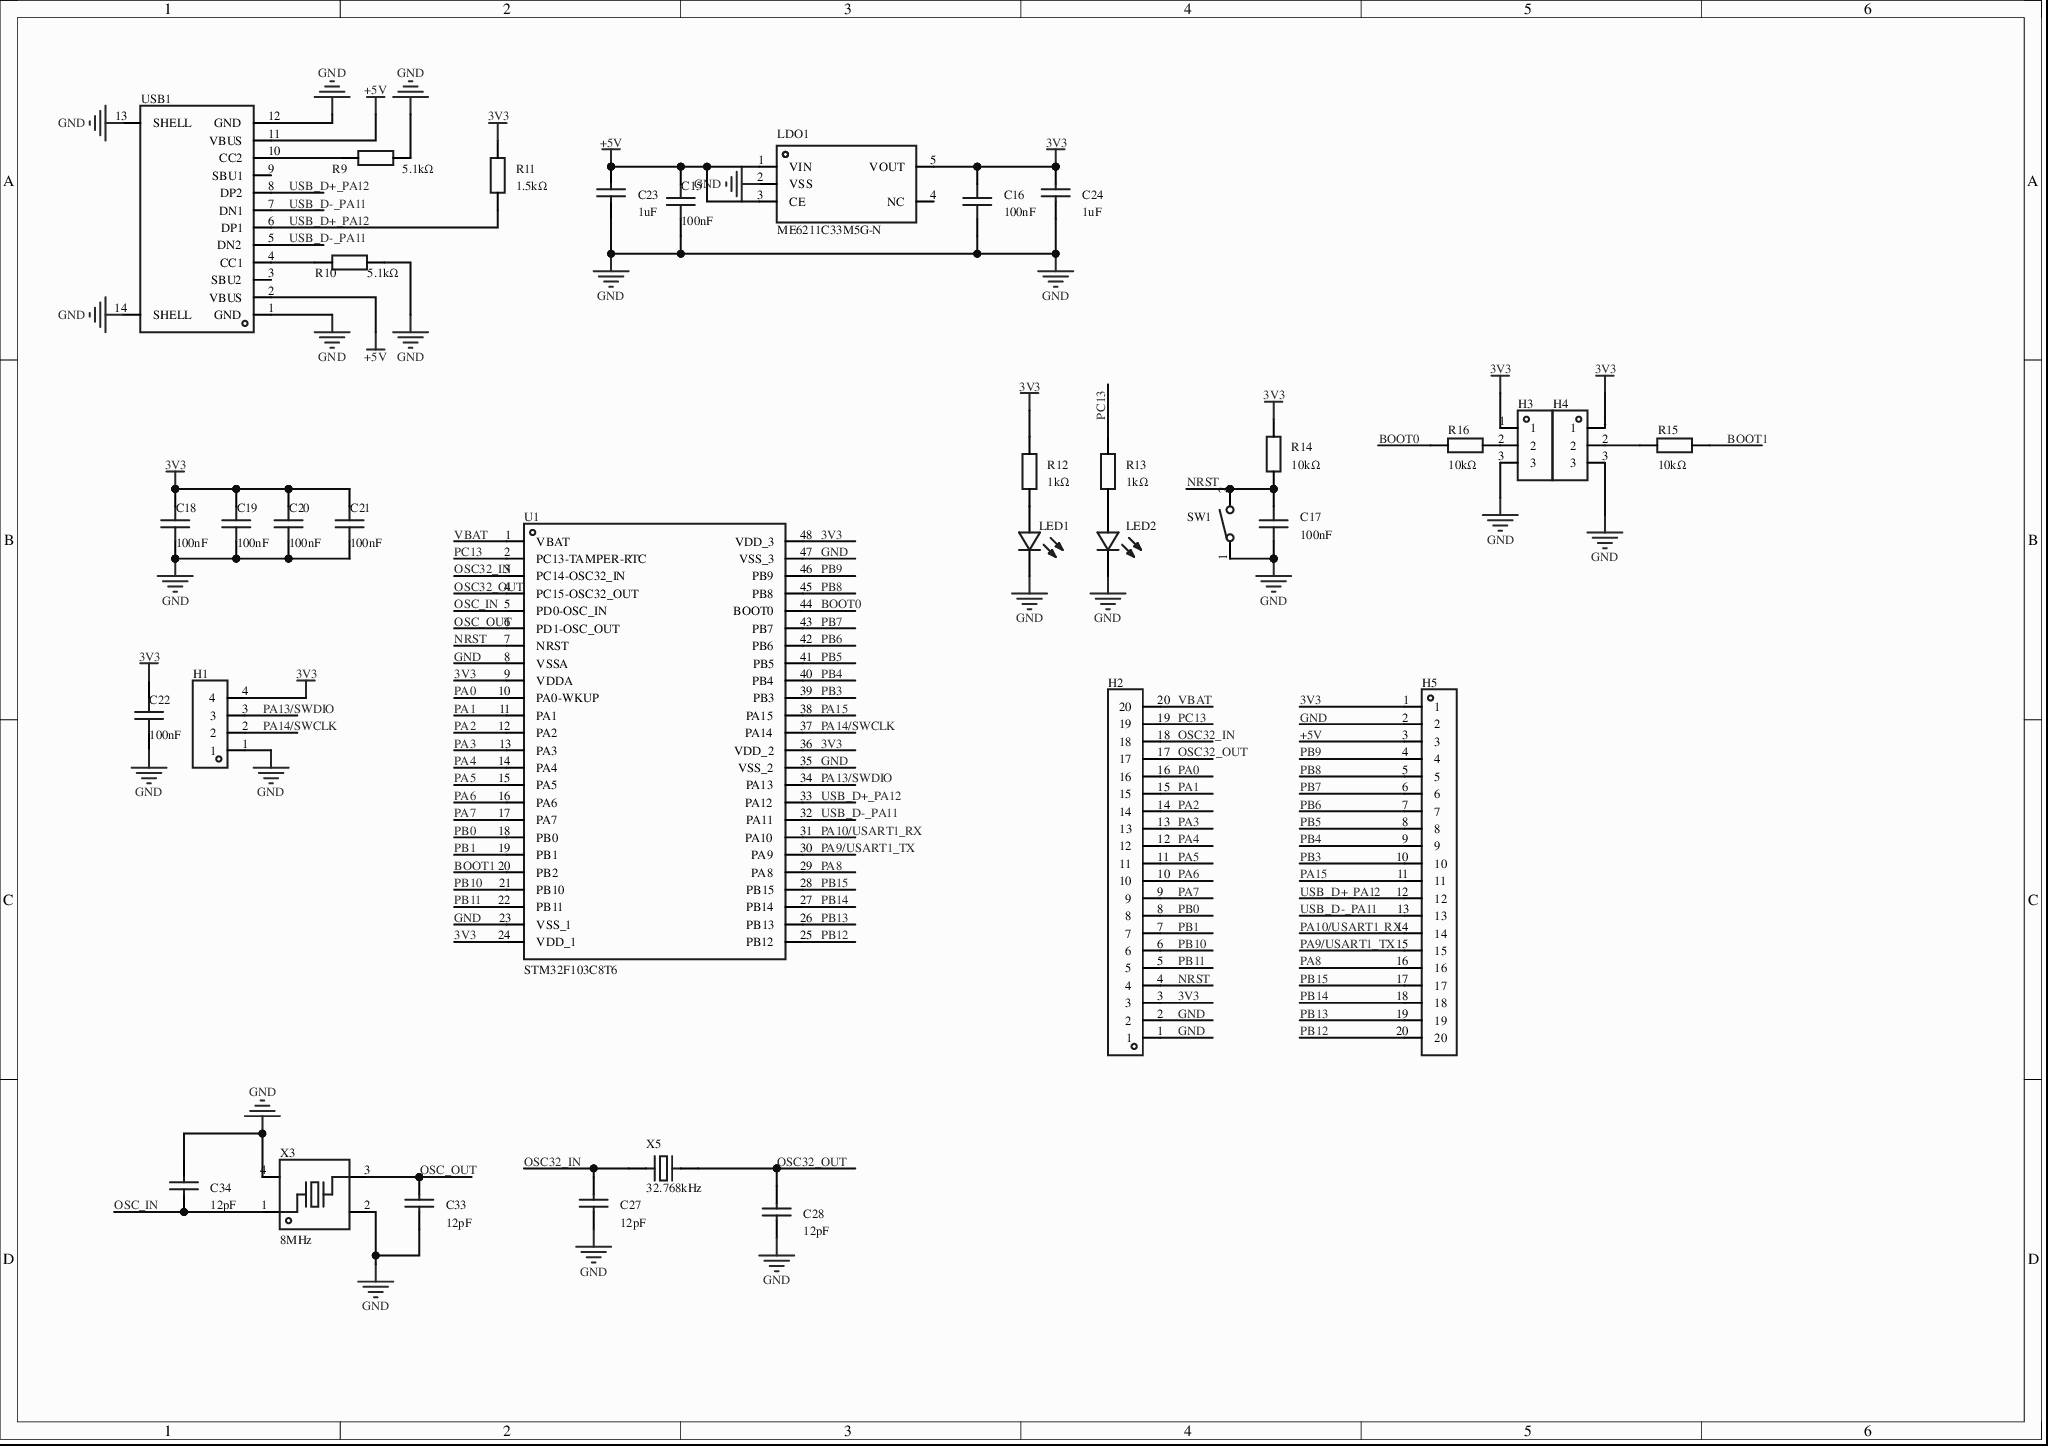
[diagram p0: MISC51884-3.schdoc]
# Altium project MISC51884-2.PrjPcb
1 sheet, 35 parts. Net scope: global (net labels, ports and power ports of the same name join across sheets).
Board file: MISC51884.pcbdoc

## Sheet MISC51884-3.schdoc
size 297 x 209 mm; Version: V1.0; @Project Name: MISC51884; @Update Date: 2026-04-17; @Create Date: 2026-04-17; @Board Name: MISC51884; @Create Time: 21:12:34; @Page Count: 1; @Page No: 1; @Schematic Name: MISC51884; @Update Time: 21:12:34; Size: A4

### Parts
C15  100nF  [C0402]
C16  100nF  [C0402]
C17  100nF  [C0402]
C18  100nF  [C0402]
C19  100nF  [C0402]
C20  100nF  [C0402]
C21  100nF  [C0402]
C22  100nF  [C0402]
C23  1uF  [C0402]
C24  1uF  [C0402]
C27  12pF  [C0402]
C28  12pF  [C0402]
C33  12pF  [C0402]
C34  12pF  [C0402]
H1  DZ254W-11-04-65  [HDR-TH_4P-P2.54-H-M-W10.3]  (value not drawn)
H2  2.54-1*20P直针  [HDR-TH_20P-P2.54-V-M-1]  (value not drawn)
H3  PZ254V-11-03P  [HDR-TH_3P-P2.54-V-M_PZ254V-11-03P]  (value not drawn)
H4  PZ254V-11-03P  [HDR-TH_3P-P2.54-V-M_PZ254V-11-03P]  (value not drawn)
H5  2.54-1*20P直针  [HDR-TH_20P-P2.54-V-M-1]  (value not drawn)
LDO1  ME6211C33M5G-N  [SOT-23-5_L3.0-W1.7-P0.95-LS2.8-BL]
LED1  NCD0603R1  [LED0603-RD_RED]  (value not drawn)
LED2  NCD0603B1  [LED0603-RD]  (value not drawn)
R9  5.1kΩ  [R0805]
R10  5.1kΩ  [R0805]
R11  1.5kΩ  [R0805]
R12  1kΩ  [R0805]
R13  1kΩ  [R0805]
R14  10kΩ  [R0805]
R15  10kΩ  [R0805]
R16  10kΩ  [R0805]
SW1  TS-1101-B-W  [KEY-SMD_2P-L6.0-W3.6-P7.4-LS8.0-L]  (value not drawn)
U1  STM32F103C8T6  [LQFP-48_L7.0-W7.0-P0.50-LS9.0-BL]
USB1  TYPE-C 16PIN 2MD(073)  [USB-C-SMD_TYPE-C-6PIN-2MD-073]  (value not drawn)
X3  8MHz  [CRYSTAL-SMD_4P-L3.2-W2.5-BL-1]
X5  32.768kHz  [OSC-SMD_L3.2-W1.5]

### Nets
3V3: C16.2 C18.2 C19.2 C20.2 C21.2 C22.2 C24.2 H1.4 H2.3 H3.1 H4.1 H5.1 LDO1.5(VOUT) R11.2 R12.2 R14.2 U1.9(VDDA) U1.24(VDD_1) U1.36(VDD_2) U1.48(VDD_3)
+5V: C15.2 C23.2 H5.3 LDO1.1(VIN) LDO1.3(CE) USB1.2(VBUS) USB1.11(VBUS)
GND: C15.1 C16.1 C17.1 C18.1 C19.1 C20.1 C21.1 C22.1 C23.1 C24.1 C27.1 C28.1 C33.1 C34.2 H1.1 H2.1 H2.2 H3.3 H4.3 H5.2 LDO1.2(VSS) LED1.1(K) LED2.1(-) R9.2 R10.2 SW1.1 U1.8(VSSA) U1.23(VSS_1) U1.35(VSS_2) U1.47(VSS_3) USB1.1(GND) USB1.12(GND) USB1.13(SHELL) USB1.14(SHELL) X3.2(GND) X3.4(GND)
BOOT0: R16.1 U1.44(BOOT0)
BOOT1: R15.2 U1.20(PB2)
NRST: C17.2 H2.4 R14.1 SW1.2 U1.7(NRST)
OSC32_IN: C27.2 H2.18 U1.3(PC14-OSC32_IN) X5.1
OSC32_OUT: C28.2 H2.17 U1.4(PC15-OSC32_OUT) X5.2
OSC_IN: C34.1 U1.5(PD0-OSC_IN) X3.1
OSC_OUT: C33.2 U1.6(PD1-OSC_OUT) X3.3
PA0: H2.16 U1.10(PA0-WKUP)
PA1: H2.15 U1.11(PA1)
PA2: H2.14 U1.12(PA2)
PA3: H2.13 U1.13(PA3)
PA4: H2.12 U1.14(PA4)
PA5: H2.11 U1.15(PA5)
PA6: H2.10 U1.16(PA6)
PA7: H2.9 U1.17(PA7)
PA8: H5.16 U1.29(PA8)
PA9/USART1_TX: H5.15 U1.30(PA9)
PA10/USART1_RX: H5.14 U1.31(PA10)
PA13/SWDIO: H1.3 U1.34(PA13)
PA14/SWCLK: H1.2 U1.37(PA14)
PA15: H5.11 U1.38(PA15)
PB0: H2.8 U1.18(PB0)
PB1: H2.7 U1.19(PB1)
PB3: H5.10 U1.39(PB3)
PB4: H5.9 U1.40(PB4)
PB5: H5.8 U1.41(PB5)
PB6: H5.7 U1.42(PB6)
PB7: H5.6 U1.43(PB7)
PB8: H5.5 U1.45(PB8)
PB9: H5.4 U1.46(PB9)
PB10: H2.6 U1.21(PB10)
PB11: H2.5 U1.22(PB11)
PB12: H5.20 U1.25(PB12)
PB13: H5.19 U1.26(PB13)
PB14: H5.18 U1.27(PB14)
PB15: H5.17 U1.28(PB15)
PC13: H2.19 R13.2 U1.2(PC13-TAMPER-RTC)
USB_D+_PA12: H5.12 R11.1 U1.33(PA12) USB1.6(DP1) USB1.8(DP2)
USB_D-_PA11: H5.13 U1.32(PA11) USB1.5(DN2) USB1.7(DN1)
VBAT: H2.20 U1.1(VBAT)
NetH3_2: H3.2 R16.2
NetH4_2: H4.2 R15.1
NetLED1_2: LED1.2(A) R12.1
NetLED2_2: LED2.2(+) R13.1
NetR9_1: R9.1 USB1.10(CC2)
NetR10_1: R10.1 USB1.4(CC1)

Not connected (* = marked no-connect by the designer): LDO1 4(NC)*; USB1 3(SBU2)* 9(SBU1)*

### Library data of the parts
C15-C22 = GRM155R71H104KE14D: 容值:100nF;精度:±10%;额定电压:50V;温度系数:X7R;; Manufacturer: muRata(村田); AddInBom: yes; ModelId: 36a51122f27c49738f86b3bfa98863e00819f05c4eef4c71ace90d822a990e87; ModelName: C0402_L1.0-W0.5-H0.5; ModelTransform: 39.37,19.685,0,0,0,0,0,0,0; Tolerance: ±10%; Voltage Rating: 50V; Temperature Coefficient: X7R; Symbol: GRM155R71H104KE14D; Device: GRM155R71H104KE14D; LCSC Part Name: 100nF ±10% 50V; SupplierPart: C77020; ManufacturerPart: GRM155R71H104KE14D; Supplier Footprint: 0402; JLCPCB Part Class: Extended Part; Datasheet: https://item.szlcsc.com/datasheet/GRM155R71H104KE14D/78147.html; Supplier: LCSC; ConvertToPcb: yes; FootprintName: C0402; Value: 100nF
C23 C24 = CL05A105KP5NNNC: 容值:1uF;精度:±10%;额定电压:10V;温度系数:X5R;; Manufacturer: SAMSUNG(三星); AddInBom: yes; ModelId: 36a51122f27c49738f86b3bfa98863e00819f05c4eef4c71ace90d822a990e87; ModelName: C0402_L1.0-W0.5-H0.5; ModelTransform: 39.37,19.685,0,0,0,0,0,0,0; Tolerance: ±10%; Voltage Rating: 10V; Temperature Coefficient: X5R; Symbol: CL05A105KP5NNNC; Device: CL05A105KP5NNNC; LCSC Part Name: 1uF ±10% 10V; SupplierPart: C14445; ManufacturerPart: CL05A105KP5NNNC; Supplier Footprint: 0402; JLCPCB Part Class: Extended Part; Datasheet: https://item.szlcsc.com/datasheet/CL05A105KP5NNNC/15107.html; Supplier: LCSC; ConvertToPcb: yes; FootprintName: C0402; Value: 1uF
C27 C28 C33 C34 = 0402CG120J500NT: 容值:12pF;精度:±5%;额定电压:50V;温度系数:C0G;; Manufacturer: FH(风华); AddInBom: yes; ModelId: 36a51122f27c49738f86b3bfa98863e00819f05c4eef4c71ace90d822a990e87; ModelName: C0402_L1.0-W0.5-H0.5; ModelTransform: 39.37,19.685,0,0,0,0,0,0,0; Tolerance: ±5%; Voltage Rating: 50V; Temperature Coefficient: C0G; Symbol: 0402CG120J500NT; Device: 0402CG120J500NT; LCSC Part Name: 12pF ±5% 50V; SupplierPart: C1547; ManufacturerPart: 0402CG120J500NT; Supplier Footprint: 0402; JLCPCB Part Class: Basic Part; Datasheet: https://item.szlcsc.com/datasheet/0402CG120J500NT/1899.html; Supplier: LCSC; ConvertToPcb: yes; FootprintName: C0402; Value: 12pF
H1 = DZ254W-11-04-65: 插针结构:1x4P;间距:2.54mm;行距:-;圆针/方针:方针;安装方式:弯插;排数:单排;总PIN位数:4P;额定电流:3A;额定电压:-;配合针长度:6mm;塑高:2.54mm;端接针长度:-;触头材质:黄铜;触头镀层:金;工作温度:-;颜色:黑色;; Manufacturer: DEALON(德艺隆); AddInBom: yes; ModelId: 380738e2c3344fc1a10fb2457d15d4660819f05c4eef4c71ace90d822a990e87; ModelTransform: 400.003,407.873,0,180,0,0,0,191.299,-118.11; Pin Structure: 1x4P; Pitch: 2.54mm; Circluar Pins/Square Pins: 方针; Current Rating: 3A; Symbol: DZ254W-11-04-65; Device: DZ254W-11-04-65; LCSC Part Name: 1x4P 间距:2.54mm 方针 弯插; SupplierPart: C2935929; ManufacturerPart: DZ254W-11-04-65; Supplier Footprint: 弯插,P=2.54mm; JLCPCB Part Class: Extended Part; Datasheet: https://item.szlcsc.com/datasheet/DZ254W-11-04-65/3287507.html; Supplier: LCSC; ConvertToPcb: yes; FootprintName: HDR-TH_4P-P2.54-H-M-W10.3; ModelName: HDR-TH_4P-P2.54-H-M-W10.3; Row Spacing: -; Mounting Type: 弯插; Number of Rows: 单排; Number of Pins: 4P; Voltage Rating (Max): -; Length of Mating Pin: 6mm; Insulation Height: 2.54mm; Length of End Connection Pin: -; Contact Material: 黄铜; Contact Plating: 金; Operating Temperature: -; Color: 黑色
H2 H5 = 2.54-1*20P直针: 插针结构:1x20P;间距:2.54mm;行距:-;圆针/方针:方针;安装方式:直插;排数:单排;总PIN位数:20P;额定电流:3A;额定电压:-;配合针长度:-;塑高:-;端接针长度:-;触头材质:黄铜;触头镀层:-;工作温度:-40℃~+105℃;颜色:黑色;; Manufacturer: BOOMELE(博穆精密); Symbol: Header-Male-2.54_1x20; AddInBom: yes; ModelId: f68709be121d406db68b06f32a5953890819f05c4eef4c71ace90d822a990e87; ModelName: HDR-M-2.54_1x20; ModelTransform: 1999.996,100,0,0,0,0,0,0,-118.11; Pin Structure: 1x20P; Pitch: 2.54mm; Circluar Pins/Square Pins: 方针; Current Rating: 3A; Device: 2.54-1*20P直针; LCSC Part Name: 1x20P 间距:2.54mm 方针 直插; SupplierPart: C50981; ManufacturerPart: 2.54-1*20P直针; Supplier Footprint: 插件,P=2.54mm; JLCPCB Part Class: Extended Part; Datasheet: https://item.szlcsc.com/datasheet/2.54-1*20P%25E7%259B%25B4%25E9%2592%2588/51993.html; Supplier: LCSC; ConvertToPcb: yes; FootprintName: HDR-TH_20P-P2.54-V-M-1; Row Spacing: -; Mounting Type: 直插; Number of Rows: 单排; Number of Pins: 20P; Voltage Rating (Max): -; Length of Mating Pin: -; Insulation Height: -; Length of End Connection Pin: -; Contact Material: 黄铜; Contact Plating: -; Operating Temperature: -40℃~+105℃; Color: 黑色
H3 H4 = PZ254V-11-03P: 插针结构:1x3P;间距:2.54mm;行距:-;圆针/方针:方针;安装方式:直插;排数:单排;总PIN位数:3P;额定电流:3A;额定电压:250V;配合针长度:6mm;塑高:2.5mm;端接针长度:3mm;工作温度:-40℃~+105℃;颜色:黑色;; Manufacturer: XFCN(兴飞); Symbol: PZ254V-11-03P_C2937625; 3D Model: bd28a638fbd247be9398fd5d39c366ec0819f05c4eef4c71ace90d822a990e87; 3D Model Transform: 300.3931,100,0,0,0,0,0,0,-118.11; Pin Structure: 1x3P; Pitch: 2.54mm; Circluar Pins/Square Pins: 方针; Current Rating: 3A; Voltage Rating (Max): 250V; AddInBom: yes; Device: PZ254V-11-03P; LCSC Part Name: 1x3P 间距:2.54mm 方针 直插; Supplier Part: C2937625; Manufacturer Part: PZ254V-11-03P; Supplier Footprint: 插件,P=2.54mm; JLCPCB Part Class: Extended Part; Datasheet: https://item.szlcsc.com/datasheet/PZ254V-11-03P/3293280.html; Supplier: LCSC; Row Spacing: -; Mounting Type: 直插; Number of Rows: 单排; Number of Pins: 3P; Length of Mating Pin: 6mm; Insulation Height: 2.5mm; Length of End Connection Pin: 3mm; Operating Temperature: -40℃~+105℃; Color: 黑色; ConvertToPcb: yes; FootprintName: HDR-TH_3P-P2.54-V-M_PZ254V-11-03P; ModelName: HDR-TH_3P-P2.54-V-M_PZ254V-11-03P
LDO1 = ME6211C33M5G-N: 输出类型:固定;工作电压:6V;输出电压:3.3V;输出电流:500mA;电源纹波抑制比(PSRR):70dB@(1kHz);输出极性:正极;; Manufacturer: MICRONE(南京微盟); 3D Model: 0a2a1b8f50944f73965918ad6e5fe1670819f05c4eef4c71ace90d822a990e87; 3D Model Transform: 118.60433,114.173,0,90,0,0,0.0005,0.0005,0; Output Type: 固定; Voltage - Supply: 6V; Output Voltage: 3.3V; Output Current: 500mA; Voltage Dropout: 120mV@(100mA); standby current: 60uA; Noise: 50uVrms; Output Configuration: 正极; Number of Outputs: 1; AddInBom: yes; ModelName: SOT-23-5_L2.9-W1.6-H1.1-LS2.8-P0.95; Symbol: ME6211C33M5G-N; Device: ME6211C33M5G-N; LCSC Part Name: 输入6V 输出3.3V 500mA; Supplier Part: C82942; Manufacturer Part: ME6211C33M5G-N; Supplier Footprint: SOT-23-5; JLCPCB Part Class: Extended Part; Datasheet: https://item.szlcsc.com/datasheet/ME6211C33M5G-N/84106.html; Supplier: LCSC; Power Supply Rejection Ratio (PSRR): 70dB@(1kHz); Features: 过流保护；带使能；短路保护; Operating Temperature: -40℃~+150℃; ConvertToPcb: yes; FootprintName: SOT-23-5_L3.0-W1.7-P0.95-LS2.8-BL
LED1 = NCD0603R1_C84263: 灯头类型:-;发光颜色:红色;正向压降(Vf):1.6V~2.6V;功率:65mW;正向电流:25mA;波长:615nm~630nm;二极管配置:独立二极管;透镜颜色:-;色温:-;发光强度:220mcd;发光角度:130°;载带方式:-;工作温度:-30℃~+85℃;; Manufacturer: 国星光电; Symbol: FC-DA1608HRK-620D; AddInBom: yes; ModelId: 74041d3a270d435c8600a9ab9b7641c00819f05c4eef4c71ace90d822a990e87; ModelTransform: 63.7794,31.496,0,0,0,0,0,-0.002,0; Illumination Color: 红色; Power(Watts): 65mW; Forward Current: 25mA; Peak Wavelength: 630nm; Diode Configuration: 独立二极管; Luminous Intensity: 220mcd; Viewing Angle: 130°; Device: NCD0603R1_C84263; LCSC Part Name: 片式发光二极管; SupplierPart: C84263; ManufacturerPart: NCD0603R1; Supplier Footprint: 0603; JLCPCB Part Class: Extended Part; Datasheet: https://item.szlcsc.com/datasheet/NCD0603R1/85432.html; Supplier: LCSC; ConvertToPcb: yes; FootprintName: LED0603-RD_RED; ModelName: LED0603-RD_RED; Lamp Holder Type: -; Voltage - Forward(Vf): 1.6V~2.6V; Wavelength - Dominant: 615nm~630nm; Lens Color: -; Color Temperature: -; Mounting Style: -; Operating Temperature: -30℃~+85℃
LED2 = NCD0603B1: 灯头类型:-;发光颜色:蓝色;正向压降(Vf):2.6V~3.6V;功率:72mW;正向电流:10mA;波长:463nm~475nm;二极管配置:独立二极管;透镜颜色:-;色温:-;发光强度:220mcd;发光角度:130°;载带方式:-;工作温度:-30℃~+85℃;; Manufacturer: 国星光电; Symbol: FC-DA1608BK-470H10; AddInBom: yes; ModelId: 1f0d29a91be547639d425604e9b96ebb0819f05c4eef4c71ace90d822a990e87; ModelTransform: 63.7794,32.283,0,0,0,0,0,0,0; Illumination Color: 蓝色; Power(Watts): 72mW; Forward Current: 10mA; Peak Wavelength: 465nm; Diode Configuration: 独立二极管; Luminous Intensity: 220mcd; Viewing Angle: 130°; Device: NCD0603B1; LCSC Part Name: 片式发光二极管; SupplierPart: C84266; ManufacturerPart: NCD0603B1; Supplier Footprint: 0603; JLCPCB Part Class: Extended Part; Datasheet: https://item.szlcsc.com/datasheet/NCD0603B1/85435.html; Supplier: LCSC; ConvertToPcb: yes; FootprintName: LED0603-RD; ModelName: LED0603-RD; Lamp Holder Type: -; Voltage - Forward(Vf): 2.6V~3.6V; Wavelength - Dominant: 463nm~475nm; Lens Color: -; Color Temperature: -; Mounting Style: -; Operating Temperature: -30℃~+85℃
R9-R16 = Res_0805: Symbol: 电阻; ConvertToPcb: yes; ModelId: 37a81e68749a4138bd2dfa6897b24b850819f05c4eef4c71ace90d822a990e87; ModelName: R0805_L2.0-W1.3-H0.6; ModelTransform: 78.74,51.181,0,0,0,0,0,-0.0005,0; Device: Res_0805; AddInBom: yes; Supplier Footprint: 0805; FootprintName: R0805
  R9 R10: Value: 5.1kΩ
  R11: Value: 1.5kΩ
  R12 R13: Value: 1kΩ
  R14-R16: Value: 10kΩ
SW1 = TS-1101-B-W_C500065: 电路结构:单刀单掷;按钮形状:矩形按钮;作用力:1.6N;安装方式:立贴;开关长度:6mm;开关宽度:3.6mm;开关高度:2.5mm;带支架:不带支架;触点电流:50mA;额定电压:12V;带灯:无;工作寿命:5万次;; Manufacturer: XKB Connection(中国星坤); AddInBom: yes; ModelId: b8d6ee452e6447ebb6dcd7a0adaffe040819f05c4eef4c71ace90d822a990e87; ModelTransform: 314.96,141.732,0,0,0,0,0,0,0; Circuit: 单刀单掷; Actuator Style: 矩形按钮; Operating Force: 1.6N; Switch Height: 2.5mm; with Bracket: 不带支架; Contact Current: 50mA; Voltage Rating: 12V; Actuator/Cap Color: 白色; With Lamp: 无; Life: 5万次; Symbol: TS-1101-B-W; Device: TS-1101-B-W_C500065; LCSC Part Name: 6*3.6*2.5mm 立贴 轻触开关; SupplierPart: C500065; ManufacturerPart: TS-1101-B-W; Supplier Footprint: SMD; JLCPCB Part Class: Extended Part; Datasheet: https://item.szlcsc.com/datasheet/TS-1101-B-W/512191.html; Supplier: LCSC; ConvertToPcb: yes; FootprintName: KEY-SMD_2P-L6.0-W3.6-P7.4-LS8.0-L; ModelName: KEY-SMD_2P-L6.0-W3.6-P7.4-LS8.0-L; Mounting Type: 立贴; Length: 6mm; Width: 3.6mm; Operating Temperature: -30℃~+85℃
U1 = STM32F103C8T6: CPU内核:ARM-M3;CPU最大主频:72MHz;应用领域:-;; Manufacturer: ST(意法半导体); AddInBom: yes; ModelId: 093be70396ff421eb2cdb946d5311efc0819f05c4eef4c71ace90d822a990e87; ModelName: LQFP-48_L7.0-W7.0-H1.4-LS9.0-P0.50; ModelTransform: 354.331,354.331,0,0,0,0,0,0,0; CPU Core: ARM-M3; CPU Maximum Speed: 72MHz; Program Storage Size: 64KB; Program Memory Type: FLASH; Number of I/O: 37; ADC (Bit): 12bit; Voltage - Supply: 2V~3.6V; Symbol: STM32F103C8T6; Device: STM32F103C8T6; LCSC Part Name: 主流增强型ARM Cortex-M3 MCU，具有64 KB Flash、72 MHz CPU、电机控制、USB和CAN; SupplierPart: C8734; ManufacturerPart: STM32F103C8T6; Supplier Footprint: LQFP-48(7x7); JLCPCB Part Class: Extended Part; Datasheet: https://item.szlcsc.com/datasheet/STM32F103C8T6/9243.html; Supplier: LCSC; ConvertToPcb: yes; FootprintName: LQFP-48_L7.0-W7.0-P0.50-LS9.0-BL; Applications: -
USB1 = TYPE-C 16PIN 2MD(073): 连接器类型:Type-C;协议标准:-;公母:母;安装方式:卧贴;触点数量:16P;端口数量:1;额定电流 - 电源:3A;工作温度:-25℃~+85℃;; Manufacturer: SHOU HAN(首韩); AddInBom: yes; ModelId: 3a41b9ec9b654a0fad4d118405ec62900819f05c4eef4c71ace90d822a990e87; ModelTransform: 351.9678,298.4246,0,0,0,0,0,-47.244,-35.433; Gender: 母; Number of Contacts: 16P; Number of Ports: 1; Current Rating-Power: 3A; Voltage Rating: 5V; Connect-Disconnect Life: 1万次; Detection color: 黑色; Symbol: TYPE-C 16PIN 2MD(073); Device: TYPE-C 16PIN 2MD(073); LCSC Part Name: Type-C 母 卧贴; SupplierPart: C2765186; ManufacturerPart: TYPE-C 16PIN 2MD(073); Supplier Footprint: SMD; JLCPCB Part Class: Extended Part; Datasheet: https://item.szlcsc.com/datasheet/TYPE-C%252016PIN%25202MD(073)/2901843.html; Supplier: LCSC; ConvertToPcb: yes; FootprintName: USB-C-SMD_TYPE-C-6PIN-2MD-073; ModelName: USB-C-SMD_TYPE-C-6PIN-2MD-073; Connector Type: Type-C; Protocol Standard: -; Mounting Type: 卧贴; Supplementary Features: -; Center Height: -; Length: -; Operating Temperature: -25℃~+85℃
X3 = XL2EL89COI-111YLC-8M: 晶振类型:贴片晶振;频率:8MHz;常温频差:±10ppm;负载电容:12pF;频率稳定度:±20ppm;; Manufacturer: YXC(扬兴晶振); AddInBom: yes; ModelId: 4495b492a02c4f389e505ec8ae3aaf1b0819f05c4eef4c71ace90d822a990e87; ModelTransform: 125.984,98.425,0,0,0,0,0,0,0; Normal temperature Frequency Tolerance: ±10ppm; Load Capacitance: 12pF; Frequency Stability: ±20ppm; Equivalent Series Resistance(ESR): 150Ω; Symbol: XL2EL89COI-111YLC-8M; Device: XL2EL89COI-111YLC-8M; LCSC Part Name: YSX321SL 8MHZ 4P 3225 12PF ±10PPM -40~85℃ (±20PPM); SupplierPart: C2973805; ManufacturerPart: XL2EL89COI-111YLC-8M; Supplier Footprint: SMD3225-4P; JLCPCB Part Class: Extended Part; Datasheet: https://item.szlcsc.com/datasheet/XL2EL89COI-111YLC-8M/3371202.html; Supplier: LCSC; ConvertToPcb: yes; FootprintName: CRYSTAL-SMD_4P-L3.2-W2.5-BL-1; ModelName: CRYSTAL-SMD_4P-L3.2-W2.5-BL-1; Type: 贴片晶振; Value: 8MHz; Operating Temperature: -40℃~+85℃
X5 = X321532768KGD2SI: 晶振类型:贴片晶振;频率:32.768kHz;常温频差:±20ppm;负载电容:12.5pF;频率稳定度:±30ppm;; Manufacturer: YXC(扬兴晶振); AddInBom: yes; ModelId: 2dd241c0893b4675b8def6f6998a82510819f05c4eef4c71ace90d822a990e87; ModelName: OSC-SMD_L3.2-W1.5-H0.8; ModelTransform: 125.984,59.055,0,0,0,0,0,0,0; Normal temperature Frequency Tolerance: ±20ppm; Load Capacitance: 12.5pF; Frequency Stability: ±30ppm; Symbol: X321532768KGD2SI; Device: X321532768KGD2SI; LCSC Part Name: YST310S 32.768KHZ 2P 3215 12.5PF ±20PPM -40~85℃; SupplierPart: C620155; ManufacturerPart: X321532768KGD2SI; Supplier Footprint: SMD3215-2P; JLCPCB Part Class: Extended Part; Datasheet: https://item.szlcsc.com/datasheet/X321532768KGD2SI/649983.html; Supplier: LCSC; ConvertToPcb: yes; FootprintName: OSC-SMD_L3.2-W1.5; Type: 贴片晶振; Value: 32.768kHz; Operating Temperature: -40℃~+85℃